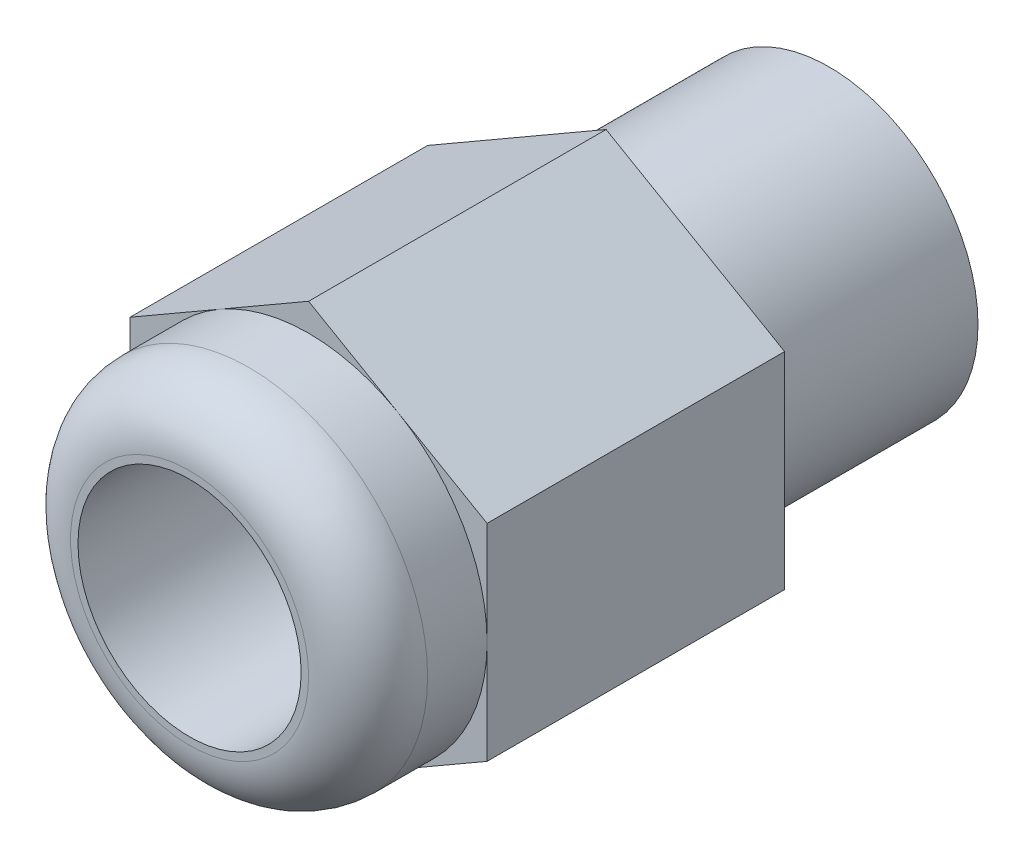
SolidWorks part; units mm, degrees
ref_plane "前视" through (0, 0, 0) normal (0, 0, 1) x (1, 0, 0)
ref_plane "上视" through (0, 0, 0) normal (0, 1, 0) x (1, 0, 0)
ref_plane "右视" through (0, 0, 0) normal (1, 0, 0) x (0, 0, -1)
sketch "草图1" plane through (0, 0, 0) normal (0, 0, 1) x (1, 0, 0)
  line L0 (0, 0) -> (0, 13.8564) construction
  line L1 (0, 13.8564) -> (-12, 6.9282)
  line L2 (-12, 6.9282) -> (-12, -6.9282)
  line L3 (-12, -6.9282) -> (0, -13.8564)
  line L4 (0, -13.8564) -> (12, -6.9282)
  line L5 (12, -6.9282) -> (12, 6.9282)
  line L6 (12, 6.9282) -> (0, 13.8564)
  circle A0 centre (0, 0) radius 12 construction
  circle A1 centre (0, 0) radius 7.5
  dimension "D1" = 15
  dimension "D2" = 24
extrude "凸台-拉伸1" add sketch "草图1" along normal blind 20
sketch "草图3" plane through (0, 0, 20) normal (0, 0, 1) x (1, 0, 0)
  circle A0 centre (0, 0) radius 12
  circle A1 centre (0, 0) radius 7.5
  circle A2 centre (0, 0) radius 7.5 construction
  dimension "D1" = 24
extrude "凸台-拉伸3" add sketch "草图3" along normal blind 8
fillet "圆角1" radius 4 1 edges at (12, 0, 28)
sketch "草图4" plane through (0, 0, 0) normal (0, 0, -1) x (-1, 0, 0)
  circle A0 centre (0, 0) radius 10
  circle A1 centre (0, 0) radius 7.5
  dimension "D1" = 20
  dimension "D2" = 15
extrude "凸台-拉伸4" add sketch "草图4" along normal blind 15
